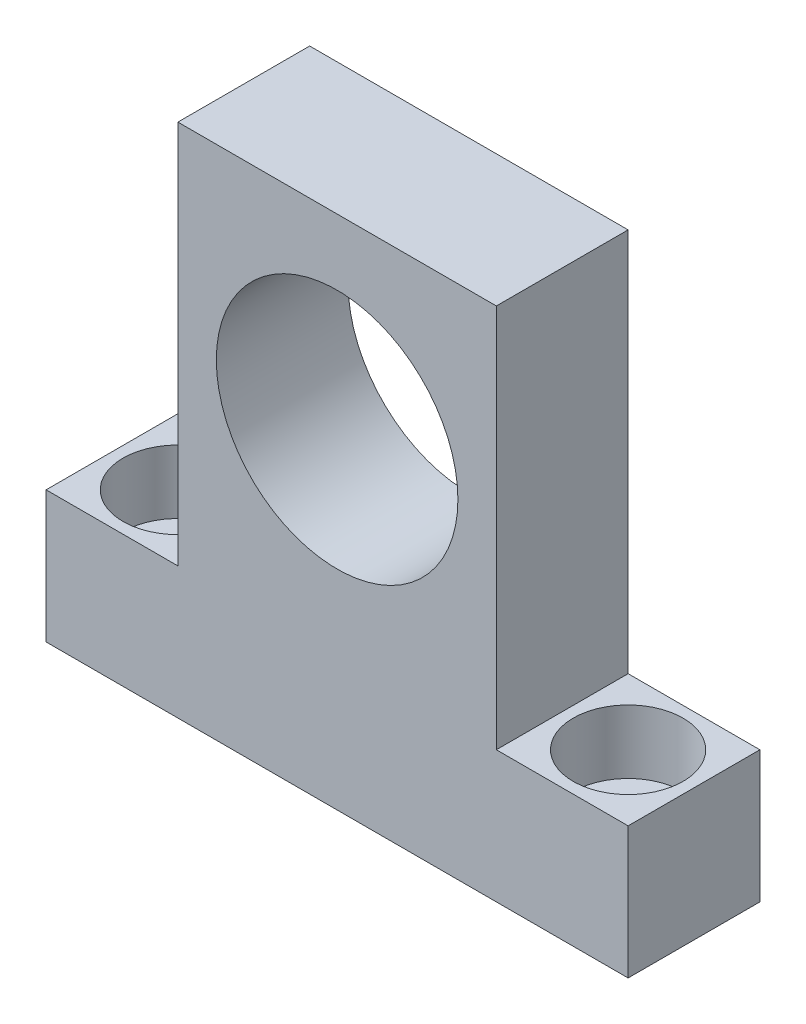
SolidWorks part; units mm, degrees
ref_plane "前视基准面" through (0, 0, 0) normal (0, 0, 1) x (1, 0, 0)
ref_plane "上视基准面" through (0, 0, 0) normal (0, 1, 0) x (1, 0, 0)
ref_plane "右视基准面" through (0, 0, 0) normal (1, 0, 0) x (0, 0, -1)
sketch "草图1" plane through (0, 0, 0) normal (0, 0, 1) x (1, 0, 0)
  line L0 (-16.2697, -16.0377) -> (36.7303, -16.0377)
  line L5 (36.7303, -16.0377) -> (36.7303, -4.0377)
  line L6 (36.7303, -4.0377) -> (24.7303, -4.0377)
  line L7 (24.7303, -4.0377) -> (24.7303, 30.9623)
  line L8 (24.7303, 30.9623) -> (-4.2697, 30.9623)
  line L9 (-4.2697, 30.9623) -> (-4.2697, -4.0377)
  line L10 (-4.2697, -4.0377) -> (-16.2697, -4.0377)
  line L11 (-16.2697, -4.0377) -> (-16.2697, -16.0377)
  circle A0 centre (10.2303, 13.9623) radius 11
  dimension "D7" = 22
  dimension "D1" = 53
  dimension "D2" = 12
  dimension "D3" = 12
  dimension "D4" = 12
  dimension "D5" = 12
  dimension "D6" = 35
  dimension "D8" = 17
  dimension "D9" = 14.5
extrude "凸台-拉伸1" add sketch "草图1" along normal blind 12
sketch "草图2" plane through (0, -4.0377, 0) normal (0, 1, 0) x (1, 0, 0)
  line L0 (-4.2697, 0) -> (-16.2697, 0) construction
  line L1 (-16.2697, -12) -> (-16.2697, 0) construction
  line L2 (36.7303, -12) -> (36.7303, 0) construction
  line L3 (36.7303, 0) -> (24.7303, 0) construction
  circle A0 centre (-10.2697, -6) radius 2.75
  circle A1 centre (30.7303, -6) radius 2.75
  dimension "D1" = 5.5
  dimension "D2" = 5.5
  dimension "D3" = 6
  dimension "D4" = 6
  dimension "D5" = 6
  dimension "D6" = 6
extrude "切除-拉伸1" cut sketch "草图2" against normal through all
sketch "草图3" plane through (0, -4.0377, 0) normal (0, 1, 0) x (1, 0, 0)
  circle A0 centre (-10.2697, -6) radius 5
  circle A1 centre (30.7303, -6) radius 5
  dimension "D1" = 10
  dimension "D2" = 10
extrude "切除-拉伸2" cut sketch "草图3" against normal blind 5.8
